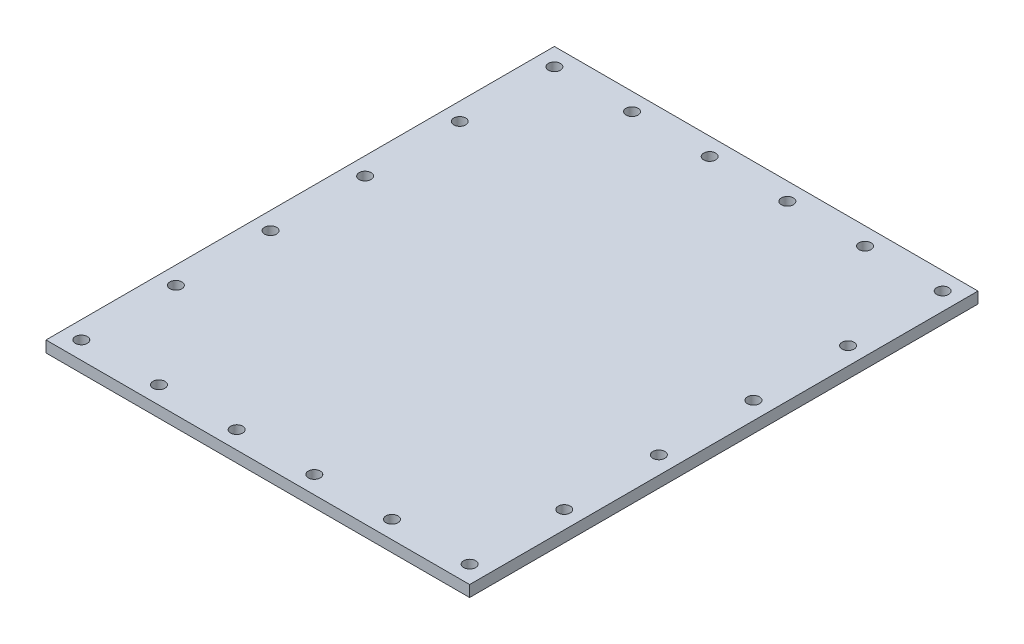
from build123d import *

# Parameters (mm, degrees)
SKETCH1_W                  = 600
SKETCH1_H                  = 720
BOSS_EXTRUDE1_DEPTH        = 8
F_17_0_17_DIAMETER_HOLE1_D = 17


with BuildPart() as part:
    # Sketch1 → Boss-Extrude1 (new, symmetric)
    with BuildSketch(Plane(origin=(0, 0, 0), x_dir=(1, 0, 0), z_dir=(0, 1, 0))):
        Rectangle(SKETCH1_W, SKETCH1_H)
    extrude(amount=BOSS_EXTRUDE1_DEPTH, both=True)

    # Ø17.0 (17) Diameter Hole1 (through all)
    with Locations(Plane(origin=(0, 8, 0), x_dir=(1, 0, 0), z_dir=(0, 1, 0))):
        with Locations((-275, -335), (-165, -335), (-55, -335), (55, -335), (165, -335), (275, -335), (-275, -201), (-275, -67), (-275, 67), (-275, 201), (-275, 335), (275, 335), (165, 335), (55, 335), (-55, 335), (-165, 335), (275, 201), (275, 67), (275, -67), (275, -201)):
            Hole(F_17_0_17_DIAMETER_HOLE1_D / 2)


solid = part.part
